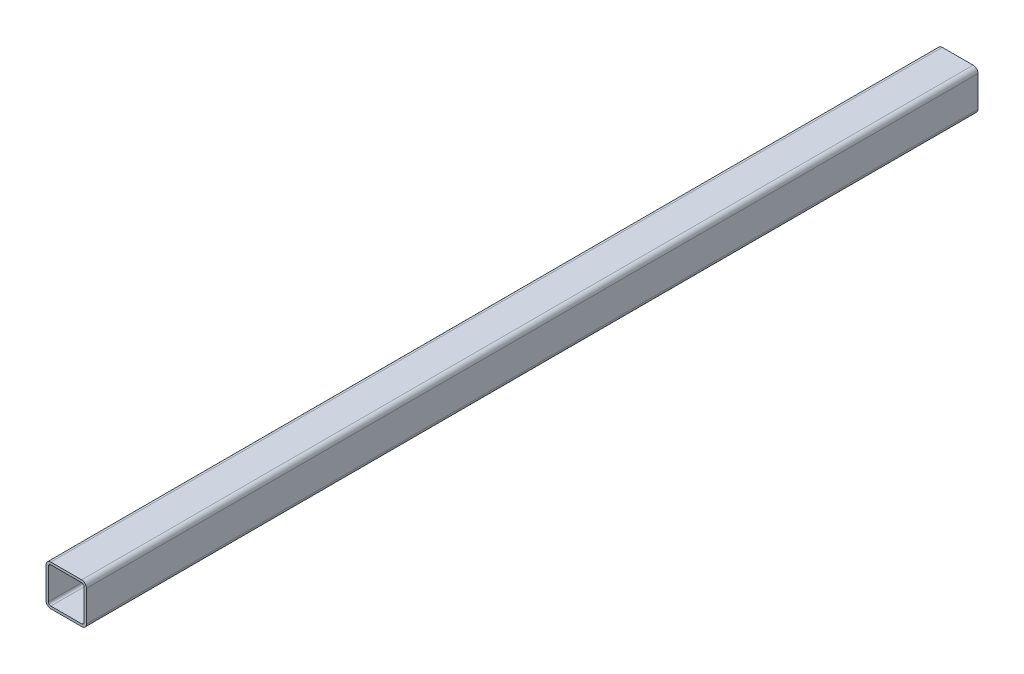
SolidWorks part; units mm, degrees
ref_plane "前视基准面" through (0, 0, 0) normal (0, 0, 1) x (1, 0, 0)
ref_plane "上视基准面" through (0, 0, 0) normal (0, 1, 0) x (1, 0, 0)
ref_plane "右视基准面" through (0, 0, 0) normal (1, 0, 0) x (0, 0, -1)
sketch "草图1" plane through (0, 0, 0) normal (0, 1, 0) x (1, 0, 0)
  line L0 (0, 0) -> (0, 1100)
  dimension "D1" = 1100
other "Gb／6728-1986方形空心型钢 050 X 50 X 3(1)"
ref_plane "基准面1" through (0, 0, 0) normal (0, 0, -1) x (-1, 0, 0)
sketch "Sketch1" plane through (0, 0, 0) normal (0, 0, -1) x (-1, 0, 0)
  line L0 (-19, -22) -> (19, -22)
  line L1 (-22, -19) -> (-22, 19)
  line L2 (19, 22) -> (-19, 22)
  line L3 (22, 19) -> (22, -19)
  line L4 (-19, -25) -> (19, -25)
  line L5 (-25, -19) -> (-25, 19)
  line L6 (19, 25) -> (-19, 25)
  line L7 (25, 19) -> (25, -19)
  arc A0 (25, 19) -> (19, 25) centre (19, 19) ccw
  arc A1 (19, -25) -> (25, -19) centre (19, -19) ccw
  arc A2 (-25, -19) -> (-19, -25) centre (-19, -19) ccw
  arc A3 (-19, 25) -> (-25, 19) centre (-19, 19) ccw
  arc A4 (-19, 22) -> (-22, 19) centre (-19, 19) ccw
  arc A5 (22, 19) -> (19, 22) centre (19, 19) ccw
  arc A6 (19, -22) -> (22, -19) centre (19, -19) ccw
  arc A7 (-22, -19) -> (-19, -22) centre (-19, -19) ccw
  point P0 (-25, 0)
  point P1 (25, 0)
  point P2 (0, 25)
  point P3 (0, -25)
  point P4 (0, 0)
  point P5 (-25, -25)
  point P6 (25, -25)
  point P7 (25, 25)
  point P8 (-25, 25)
  point P33 (0, 0)
  dimension "D1" = 6
  dimension "Thickness" = 3
  dimension "V_leg" = 50
hole_wizard "M6 螺纹孔1" positions "草图2" profile "草图3" tap size "M6" standard "GB"
sketch "草图2" plane through (0, -25, 0) normal (0, -1, 0) x (-1, 0, 0)
  point P0 (-5, 100)
  point P3 (-5, 400)
  point P6 (-5, 700)
  point P9 (-5, 1000)
sketch "草图3" plane through (5, -25, -100) normal (1, 0, 0) x (0, 0, -1)
  line L0 (0, 0) -> (0, 16.5022)
  line L1 (0, 16.5022) -> (2.5, 15)
  line L2 (2.5, 15) -> (2.5, 0)
  line L5 (2.5, 0) -> (0, 0)
  line L10 (0, 16.5022) -> (-2.5, 15) construction
  line L11 (0, -6.35) -> (0, 107.95) construction
  dimension "螺纹孔钻头直径" = 5
  dimension "螺纹孔钻头深度" = 15
  dimension "导头角度" = 118
cosmetic thread "孔螺蚊线1" parameters "D1"=3, "D2"=6
cosmetic thread "孔螺蚊线2" parameters "D1"=3, "D2"=6
cosmetic thread "孔螺蚊线3" parameters "D1"=3, "D2"=6
cosmetic thread "孔螺蚊线4" parameters "D1"=3, "D2"=6
